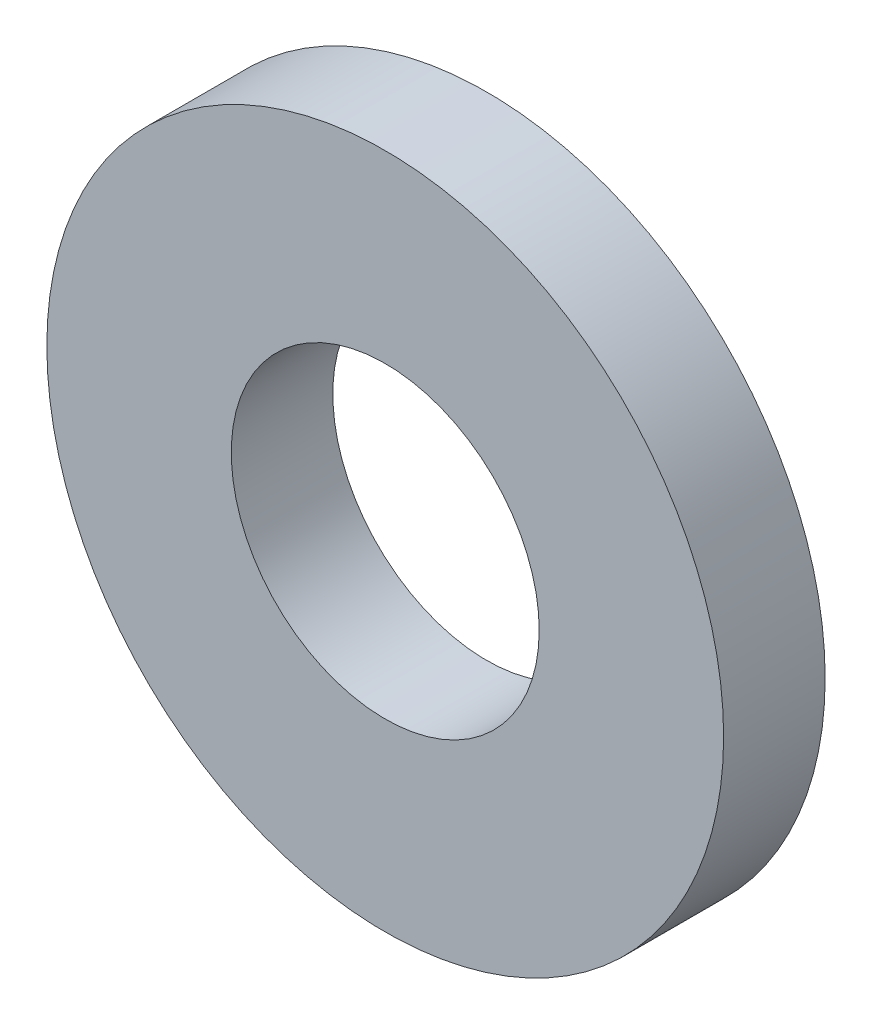
SolidWorks part; units mm, degrees
ref_plane "前视" through (0, 0, 0) normal (0, 0, 1) x (1, 0, 0)
ref_plane "上视" through (0, 0, 0) normal (0, 1, 0) x (1, 0, 0)
ref_plane "右视" through (0, 0, 0) normal (1, 0, 0) x (0, 0, -1)
sketch "草图1" plane through (0, 0, 0) normal (0, 0, 1) x (1, 0, 0)
  circle A0 centre (0, 0) radius 50
  circle A1 centre (0, 0) radius 22.75
extrude "凸台-拉伸1" add sketch "草图1" along normal blind 15
